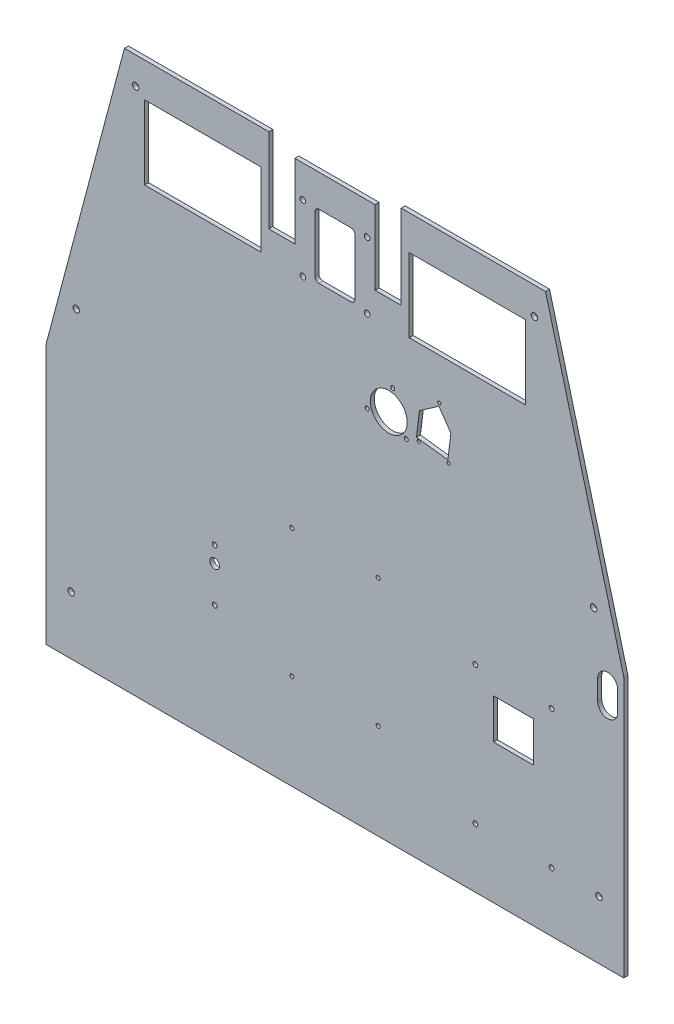
SolidWorks part; units mm, degrees
material "Rubber"
ref_plane "Front Plane" through (0, 0, 0) normal (0, 0, 1) x (1, 0, 0)
ref_plane "Top Plane" through (0, 0, 0) normal (0, 1, 0) x (1, 0, 0)
ref_plane "Right Plane" through (0, 0, 0) normal (1, 0, 0) x (0, 0, -1)
sketch "Sketch1" plane through (0, 0, 0) normal (0, 0, 1) x (1, 0, 0)
  line L0 (0, -12743.2508) -> (0, 624419.2913) construction
  line L1 (-12743.2508, 0) -> (624419.2913, 0) construction
  line L2 (-720, 0) -> (720, 0)
  line L3 (720, 0) -> (720, 650)
  line L4 (720, 650) -> (525, 1385)
  line L5 (525, 1385) -> (-525, 1385)
  line L6 (-525, 1385) -> (-720, 650)
  line L7 (-720, 650) -> (-720, 0)
  dimension "D1" = 1440
  dimension "D2" = 650
  dimension "D3" = 1385
  dimension "D4" = 1050
extrude "Boss-Extrude1" add sketch "Sketch1" along normal blind 10
sketch "Sketch2" plane through (0, 0, 10) normal (0, 0, 1) x (1, 0, 0)
  line L0 (-720, 0) -> (720, 0) construction
  circle A0 centre (-658, 145) radius 8
  dimension "D1" = 16
  dimension "D2" = 145
  dimension "D3" = 658
extrude "Cut-Extrude1" cut sketch "Sketch2" against normal blind 10
pattern_linear "LPattern1" count 2 spacing 1316 along (1, 0, 0) of "Cut-Extrude1"
sketch "Sketch3" plane through (0, 0, 10) normal (0, 0, 1) x (1, 0, 0)
  line L0 (-720, 0) -> (720, 0) construction
  circle A0 centre (-645, 762) radius 8
  dimension "D1" = 16
  dimension "D2" = 762
  dimension "D3" = 645
extrude "Cut-Extrude2" cut sketch "Sketch3" against normal blind 10
pattern_linear "LPattern2" count 2 spacing 1290 along (1, 0, 0) of "Cut-Extrude2"
sketch "Sketch4" plane through (0, 0, 10) normal (0, 0, 1) x (1, 0, 0)
  line L0 (-720, 0) -> (720, 0) construction
  circle A0 centre (-497, 1317) radius 8
  dimension "D1" = 16
  dimension "D2" = 1317
  dimension "D3" = 497
extrude "Cut-Extrude3" cut sketch "Sketch4" against normal blind 10
pattern_linear "LPattern3" count 2 spacing 994 along (1, 0, 0) of "Cut-Extrude3"
sketch "Sketch5" plane through (0, 0, 10) normal (0, 0, 1) x (1, 0, 0)
  line L0 (-720, 0) -> (720, 0) construction
  line L1 (720, 0) -> (720, 650) construction
  line L2 (655, 615) -> (655, 565)
  line L3 (705, 615) -> (705, 565)
  arc A0 (655, 565) -> (705, 565) centre (680, 565) ccw
  arc A1 (705, 615) -> (655, 615) centre (680, 615) ccw
  dimension "D4" = 25
  dimension "D1" = 565
  dimension "D2" = 50
  dimension "D3" = 40
extrude "Cut-Extrude4" cut sketch "Sketch5" against normal blind 10
sketch "Sketch6" plane through (0, 0, 10) normal (0, 0, 1) x (1, 0, 0)
  line L0 (720, 0) -> (720, 650) construction
  line L1 (395, 447) -> (495, 447)
  line L2 (395, 447) -> (395, 347)
  line L3 (395, 347) -> (495, 347)
  line L4 (495, 447) -> (495, 347)
  line L5 (-720, 0) -> (720, 0) construction
  dimension "D1" = 225
  dimension "D2" = 347
  dimension "D3" = 100
  dimension "D4" = 100
extrude "Cut-Extrude5" cut sketch "Sketch6" against normal blind 10
sketch "Sketch7" plane through (0, 0, 10) normal (0, 0, 1) x (1, 0, 0)
  line L0 (720, 0) -> (720, 650) construction
  line L1 (-720, 0) -> (720, 0) construction
  circle A0 centre (540, 492) radius 6
  dimension "D1" = 12
  dimension "D2" = 180
  dimension "D3" = 492
extrude "Cut-Extrude6" cut sketch "Sketch7" against normal blind 10
pattern_linear "LPattern4" count 2 spacing 190 along (-1, 0, 0) count 2 spacing 344 along (0, -1, 0) of "Cut-Extrude6"
sketch "Sketch8" plane through (0, 0, 10) normal (0, 0, 1) x (1, 0, 0)
  line L0 (-720, 0) -> (720, 0) construction
  circle A0 centre (107.5, 238) radius 5
  dimension "D1" = 10
  dimension "D2" = 107.5
  dimension "D3" = 238
extrude "Cut-Extrude7" cut sketch "Sketch8" against normal blind 10
pattern_linear "LPattern5" count 2 spacing 320 along (0, 1, 0) count 2 spacing 215 along (-1, 0, 0) of "Cut-Extrude7"
sketch "Sketch9" plane through (0, 0, 10) normal (0, 0, 1) x (1, 0, 0)
  line L0 (525, 1385) -> (-525, 1385) construction
  line L1 (-475, 1299) -> (-185, 1299)
  line L2 (-475, 1299) -> (-475, 1115)
  line L4 (-475, 1115) -> (-185, 1115)
  line L5 (-185, 1299) -> (-185, 1115)
  dimension "D3" = 270
  dimension "D1" = 185
  dimension "D2" = 290
  dimension "D4" = 184
extrude "Cut-Extrude8" cut sketch "Sketch9" against normal blind 10
sketch "Sketch10" plane through (0, 0, 10) normal (0, 0, 1) x (1, 0, 0)
  line L0 (0, -1000) -> (0, 49000) construction
  line L1 (525, 1385) -> (-525, 1385) construction
  line L2 (-50, 1280) -> (50, 1280)
  line L3 (-50, 1280) -> (-50, 1120)
  line L4 (-50, 1120) -> (50, 1120)
  line L5 (50, 1280) -> (50, 1120)
  dimension "D1" = 105
  dimension "D2" = 160
  dimension "D3" = 100
extrude "Cut-Extrude9" cut sketch "Sketch10" against normal blind 10
fillet "Fillet1" radius 10 4 edges at (50, 1120, 5) (-50, 1120, 5) (50, 1280, 5) (-50, 1280, 5)
sketch "Sketch11" plane through (0, 0, 10) normal (0, 0, 1) x (1, 0, 0)
  line L0 (525, 1385) -> (-525, 1385) construction
  circle A0 centre (80, 1280) radius 7
  dimension "D1" = 14
  dimension "D2" = 80
  dimension "D3" = 105
extrude "Cut-Extrude10" cut sketch "Sketch11" against normal blind 10
pattern_linear "LPattern7" count 2 spacing 160 along (-1, 0, 0) count 2 spacing 165 along (0, -1, 0) of "Cut-Extrude10"
sketch "Sketch12" plane through (0, 0, 10) normal (0, 0, 1) x (1, 0, 0)
  line L0 (525, 1385) -> (-525, 1385) construction
  circle A0 centre (144, 986) radius 5
  dimension "D1" = 10
  dimension "D2" = 399
  dimension "D3" = 144
extrude "Cut-Extrude11" cut sketch "Sketch12" against normal blind 10
sketch "Sketch14" plane through (0, 0, 10) normal (0, 0, 1) x (1, 0, 0)
  line L0 (0, -1000) -> (0, 49000) construction
  line L1 (144, 986) -> (-8538.4089, -48254.3877) construction
  circle A0 centre (134.0673, 929.669) radius 46
  point P6 (144, 986)
  dimension "D3" = 92
  dimension "D1" = 10
  dimension "D2" = 57.2
extrude "Cut-Extrude12" cut sketch "Sketch14" against normal blind 10
sketch "Sketch15" plane through (0, 0, 10) normal (0, 0, 1) x (1, 0, 0)
  line L0 (144, 986) -> (129.0663, 901.3065) construction
  line L1 (36.8819, 917.5611) -> (204.7665, 887.9585) construction
  line L2 (0, -1000) -> (0, 49000) construction
  circle A0 centre (80.3183, 909.9021) radius 5
  dimension "D3" = 10
  dimension "D1" = 90
  dimension "D2" = 86
  dimension "D4" = 49.5
  dimension "D5" = 10
extrude "Cut-Extrude13" cut sketch "Sketch15" against normal blind 10
pattern_linear "LPattern8" count 2 spacing 99 along (0.9848, -0.1736, 0) of "Cut-Extrude13"
sketch "Sketch16" plane through (0, 0, 10) normal (0, 0, 1) x (1, 0, 0)
  line L0 (525, 1385) -> (-525, 1385) construction
  circle A0 centre (260, 1012) radius 4
  dimension "D3" = 8
  dimension "D1" = 260
  dimension "D2" = 373
extrude "Cut-Extrude14" cut sketch "Sketch16" against normal blind 10
sketch "Sketch17" plane through (0, 0, 10) normal (0, 0, 1) x (1, 0, 0)
  line L0 (0, -1000) -> (0, 49000) construction
  line L1 (260, 1012) -> (-5833.4672, -48615.3076) construction
  line L2 (259.025, 1004.0596) -> (210.5705, 970.4716)
  line L3 (259.025, 1004.0596) -> (288.9817, 960.8439)
  line L4 (210.5705, 970.4716) -> (203.0442, 909.1747)
  line L5 (288.9817, 960.8439) -> (281.4554, 899.547)
  line L6 (281.4554, 899.547) -> (203.0442, 909.1747)
  point P6 (260, 1012)
  dimension "D1" = 7
  dimension "D2" = 109
  dimension "D3" = 79
  dimension "D4" = 44
  dimension "D5" = 8
extrude "Cut-Extrude15" cut sketch "Sketch17" against normal blind 10
sketch "Sketch18" plane through (0, 0, 10) normal (0, 0, 1) x (1, 0, 0)
  line L0 (0, -1000) -> (0, 49000) construction
  line L1 (260, 1012) -> (-5833.4672, -48615.3076) construction
  line L2 (208.7645, 902.4273) -> (280.1734, 893.6594) construction
  circle A0 centre (208.7645, 902.4273) radius 4
  circle A2 centre (260, 1012) radius 4 construction
  dimension "D2" = 8
  dimension "D1" = 7
  dimension "D3" = 37.5
  dimension "D4" = 90
  dimension "D5" = 115
extrude "Cut-Extrude16" cut sketch "Sketch18" against normal blind 10
pattern_linear "LPattern9" count 2 spacing 75 along (0.9925, -0.1219, 0) of "Cut-Extrude16"
sketch "Sketch19" plane through (0, 0, 10) normal (0, 0, 1) x (1, 0, 0)
  line L0 (-720, 0) -> (720, 0) construction
  circle A0 centre (-300, 295) radius 6
  dimension "D3" = 12
  dimension "D1" = 300
  dimension "D2" = 295
extrude "Cut-Extrude17" cut sketch "Sketch19" against normal blind 10
pattern_linear "LPattern10" count 2 spacing 130 along (0, 1, 0) of "Cut-Extrude17"
sketch "Sketch20" plane through (0, 0, 10) normal (0, 0, 1) x (1, 0, 0)
  line L0 (-720, 0) -> (720, 0) construction
  circle A0 centre (-300, 385) radius 12
  dimension "D3" = 24
  dimension "D1" = 300
  dimension "D2" = 385
extrude "Cut-Extrude18" cut sketch "Sketch20" against normal blind 10
pattern_linear "LPattern11" count 2 spacing 660 along (1, 0, 0) of "Cut-Extrude8"
sketch "Sketch21" plane through (0, 0, 10) normal (0, 0, 1) x (1, 0, 0)
  line L0 (525, 1385) -> (-525, 1385) construction
  line L1 (100, 1385) -> (165, 1385)
  line L2 (100, 1385) -> (100, 1175)
  line L3 (100, 1175) -> (165, 1175)
  line L4 (165, 1385) -> (165, 1175)
  dimension "D1" = 100
  dimension "D2" = 165
  dimension "D3" = 210
extrude "Cut-Extrude19" cut sketch "Sketch21" against normal blind 10
sketch "Sketch22" plane through (0, 0, 10) normal (0, 0, 1) x (1, 0, 0)
  line L0 (100, 1385) -> (-525, 1385) construction
  line L1 (-165, 1385) -> (-100, 1385)
  line L2 (-165, 1385) -> (-165, 1175)
  line L3 (-165, 1175) -> (-100, 1175)
  line L4 (-100, 1385) -> (-100, 1175)
  dimension "D1" = 100
  dimension "D2" = 165
  dimension "D3" = 210
extrude "Cut-Extrude20" cut sketch "Sketch22" against normal blind 10
sketch "Sketch23" plane through (0, 0, 10) normal (0, 0, 1) x (1, 0, 0)
  line L0 (100, 1385) -> (100, 1175) construction
  line L1 (-100, 1385) -> (100, 1385)
  line L2 (-100, 1385) -> (-100, 1360)
  line L3 (-100, 1360) -> (100, 1360)
  line L4 (100, 1385) -> (100, 1360)
  line L5 (100, 1175) -> (165, 1175) construction
  dimension "D1" = 185
extrude "Cut-Extrude21" cut sketch "Sketch23" against normal blind 10
